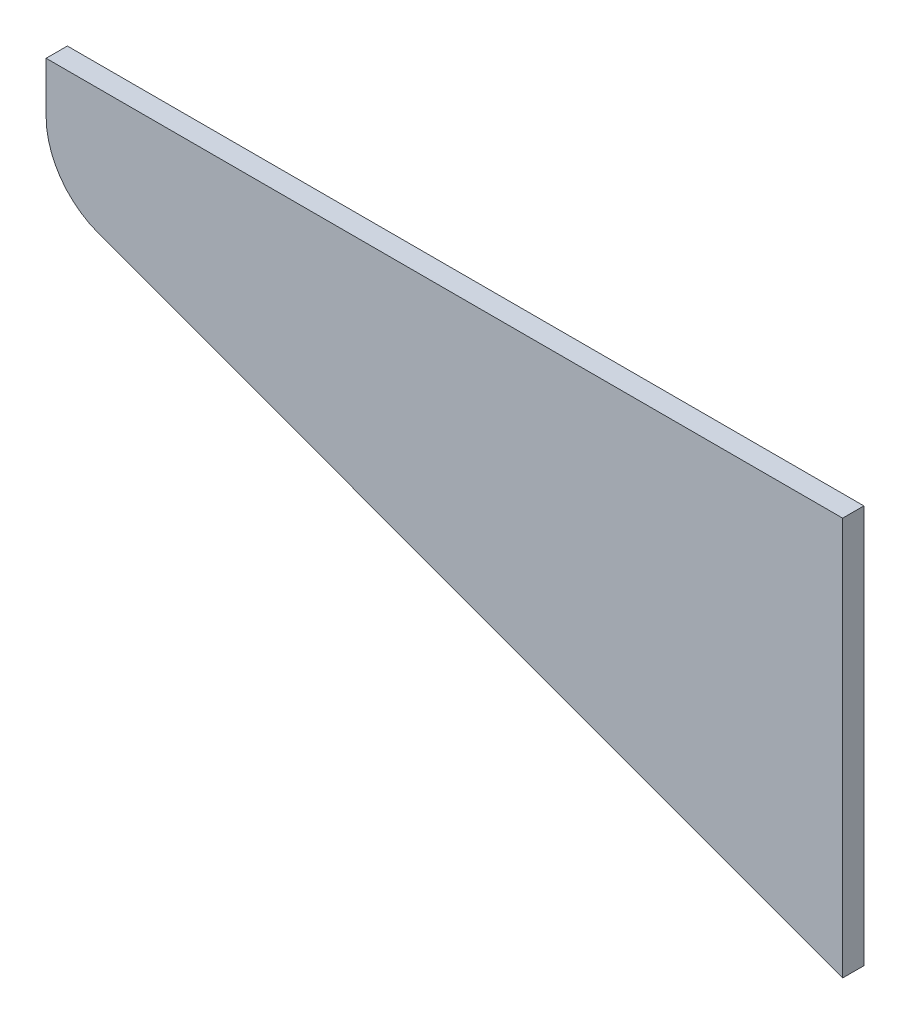
from build123d import *

# Parameters (mm, degrees)
EXTRUDE_2_DEPTH = 8


with BuildPart() as part:
    # 草图1 → 凸台-拉伸2 (new body)
    with BuildSketch(Plane.XY):
        with BuildLine():
            Line((330, 0), (30, 0))
            Line((30, 0), (30, -19.046909383))
            ThreePointArc((30, -19.046909383), (35.404988471, -36.22495956), (49.672360525, -47.213198859))
            Line((49.672360525, -47.213198859), (330, -150))
            Line((330, -150), (330, 0))
        make_face()
    extrude(amount=EXTRUDE_2_DEPTH)


solid = part.part
